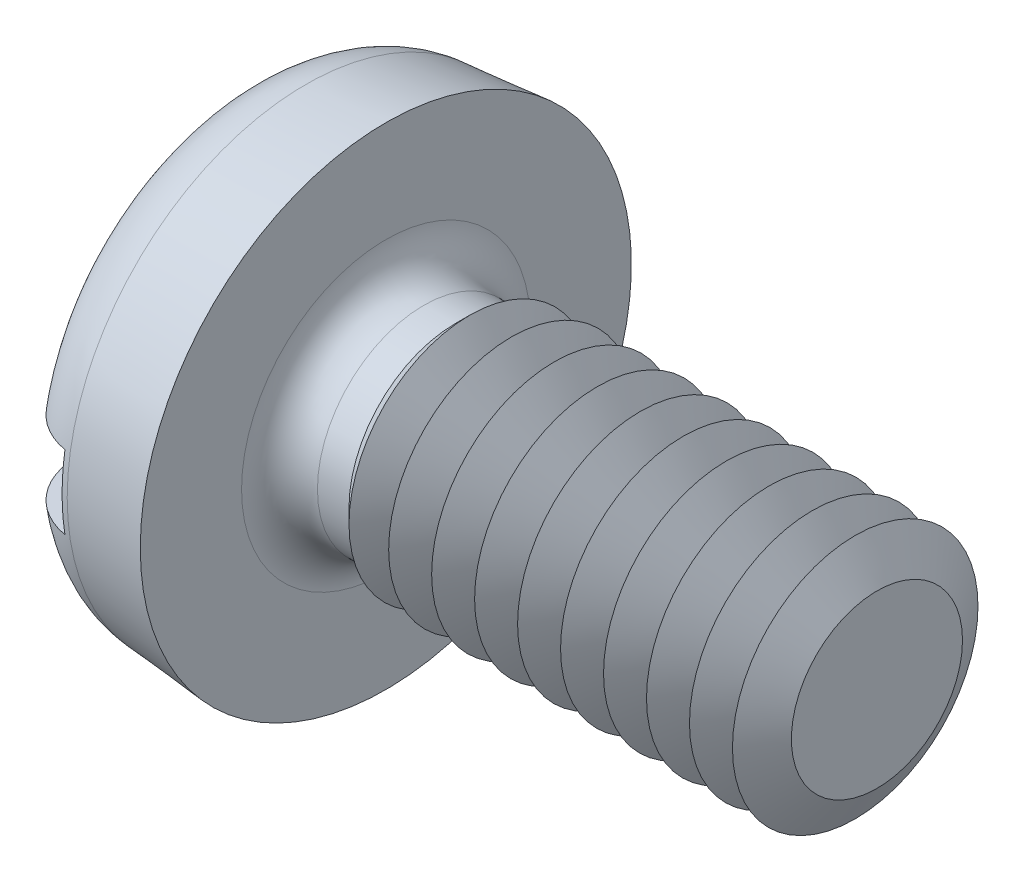
SolidWorks part; units mm, degrees
revolve "基体-旋转" add sketch "草图3" angle 360 about L0
sketch "草图3" plane through (0, 0, 0) normal (0, 0, 1) x (1, 0, 0)
  line L0 (-2.477, 0) -> (6.7868, 0) construction
  line L1 (0, 0) -> (10.4, 0)
  line L2 (10.4, 0) -> (10.4, 2)
  line L3 (10.4, 2) -> (3.8, 2)
  line L4 (2.4, 2.35) -> (2.4, 4)
  line L5 (3.8, 2) -> (3.532, 1.732)
  line L6 (3.532, 1.732) -> (3.018, 1.732)
  line L7 (2.4, 4) -> (1.0954, 3.8859)
  line L9 (0, 2.6904) -> (0, 0)
  arc A0 (3.018, 1.732) -> (2.4, 2.35) centre (3.018, 2.35) cw
  arc A1 (1.0954, 3.8859) -> (0, 2.6904) centre (1.2, 2.6904) ccw
cosmetic thread "装饰螺纹线1" parameters "D1"=6.6, "D2"=3.464
ref_plane "前视" through (0, 0, 0) normal (0, 0, 1) x (1, 0, 0)
ref_plane "上视" through (0, 0, 0) normal (0, 1, 0) x (1, 0, 0)
ref_plane "右视" through (0, 0, 0) normal (1, 0, 0) x (0, 0, -1)
sketch "尺寸草图" plane through (0, 0, 0) normal (0, 0, 1) x (1, 0, 0)
  line L0 (0, 0) -> (8, 0)
  line L1 (0, 0) -> (0, 8)
  line L2 (8, 0) -> (8, 4.7)
  point P5 (7.3, 0)
  point P6 (2.4, 0)
  point P7 (1.2, 0)
  point P8 (1.4, 0)
  point P9 (8, 0.2)
  point P10 (6.8, 0)
  point P11 (0, 1)
  point P12 (8, 4)
sketch "草图4" plane through (0, 0, 0) normal (0, 0, 1) x (1, 0, 0)
  line L0 (0, 2.6904) -> (0, -2.6904) construction
  line L1 (0, 0.6) -> (1, 0.6)
  line L2 (0, 0.6) -> (0, -0.6)
  line L3 (0, -0.6) -> (1, -0.6)
  line L4 (1, 0.6) -> (1, -0.6)
  point P6 (0, 0)
extrude "切除-拉伸1" cut sketch "草图4" against normal mid plane 100
sketch "草图5" plane through (0, 0, 0) normal (0, 0, 1) x (1, 0, 0)
  line L0 (10.0462, 2) -> (10.7462, 2)
  line L1 (10.7462, 2) -> (10.4, 1.3938)
  line L2 (10.4, 1.3938) -> (10.0462, 2)
  line L3 (10.4, 2) -> (3.8, 2) construction
  line L4 (10.4, -2) -> (10.4, 2) construction
  line L5 (6.175, 0) -> (-0.2582, 0) construction
  line L6 (-2.477, 0) -> (6.7868, 0) construction
revolve "切除-旋转1" cut sketch "草图5" angle 360 about L5
pattern_linear "阵列(线性)1" count 10 spacing 0.7 along (-1, 0, 0) of "切除-旋转1"
equation "\"l@草图3\" = \"l@尺寸草图\""
equation "\"dk@草图3\"=\"dk@尺寸草图\""
equation "\"da@草图3\" = \"da@尺寸草图\""
equation "\"D3@草图3\" = \"d@尺寸草图\"*0.866"
equation "\"D4@草图3\" = \"l@尺寸草图\"-\"a@尺寸草图\""
equation "\"d@草图3\" = \"d@尺寸草图\""
equation "\"D2@装饰螺纹线1\" = \"d@尺寸草图\"*0.866"
equation "\"D1@装饰螺纹线1\" = \"l@尺寸草图\"-\"a@尺寸草图\""
equation "\"n@草图4\" = \"n@尺寸草图\""
equation "\"t@草图4\" = \"t@尺寸草图\""
equation "\"P@草图5\" = \"P@尺寸草图\""
equation "\"D1@草图5\" = \"P@草图5\"*0.866"
equation "\"D3@阵列(线性)1\" = \"P@尺寸草图\""
equation "\"D1@阵列(线性)1\" = (\"l@尺寸草图\"-\"a@尺寸草图\")/\"P@尺寸草图\"+1"
equation "\"k@草图3\"=\"k@尺寸草图\""
equation "\"D5@草图3\"=\"rf@尺寸草图\""
